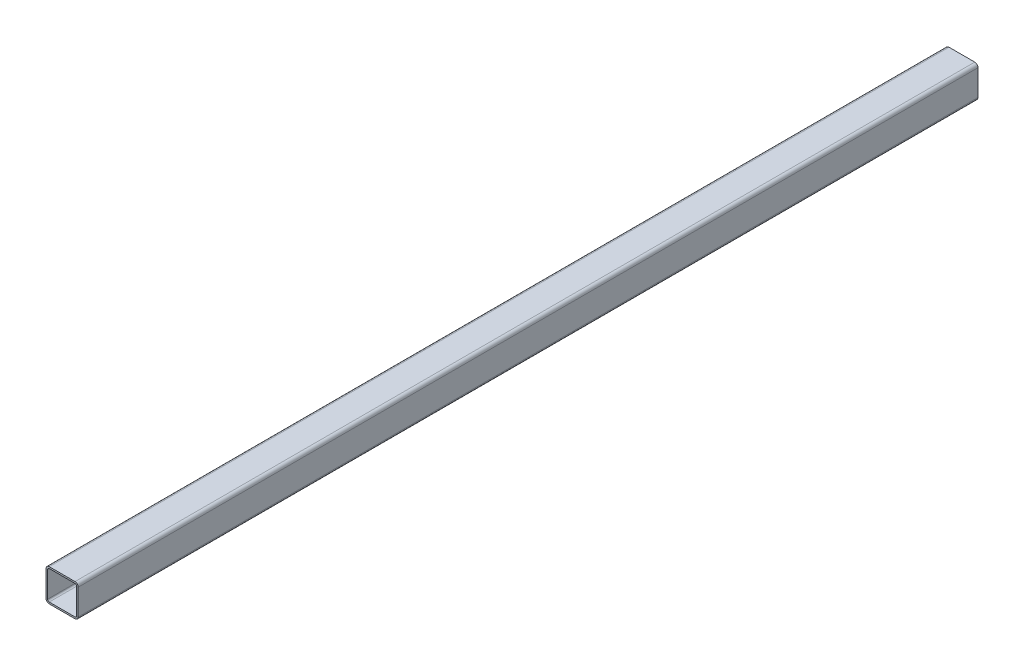
from build123d import *

# Parameters (mm, degrees)
SKETCH1_W           = 40
SKETCH1_H           = 40
SKETCH1_W_2         = 36
SKETCH1_H_2         = 36
BOSS_EXTRUDE1_DEPTH = 1116
FILLET1_R           = 2
FILLET2_R           = 4


with BuildPart() as part:
    # Sketch1 → Boss-Extrude1 (new body)
    with BuildSketch(Plane.XY):
        Rectangle(SKETCH1_W, SKETCH1_H)
        Rectangle(SKETCH1_W_2, SKETCH1_H_2, mode=Mode.SUBTRACT)
    extrude(amount=BOSS_EXTRUDE1_DEPTH)

    # Fillet1
    fillet1_edges = [part.edges().sort_by_distance(p)[0] for p in [
        (18, -18, 558),
        (18, 18, 558),
        (-18, 18, 558),
        (-18, -18, 558),
    ]]
    fillet(fillet1_edges, radius=FILLET1_R)

    # Fillet2
    fillet2_edges = [part.edges().sort_by_distance(p)[0] for p in [
        (20, -20, 558),
        (-20, -20, 558),
        (-20, 20, 558),
        (20, 20, 558),
    ]]
    fillet(fillet2_edges, radius=FILLET2_R)


solid = part.part
